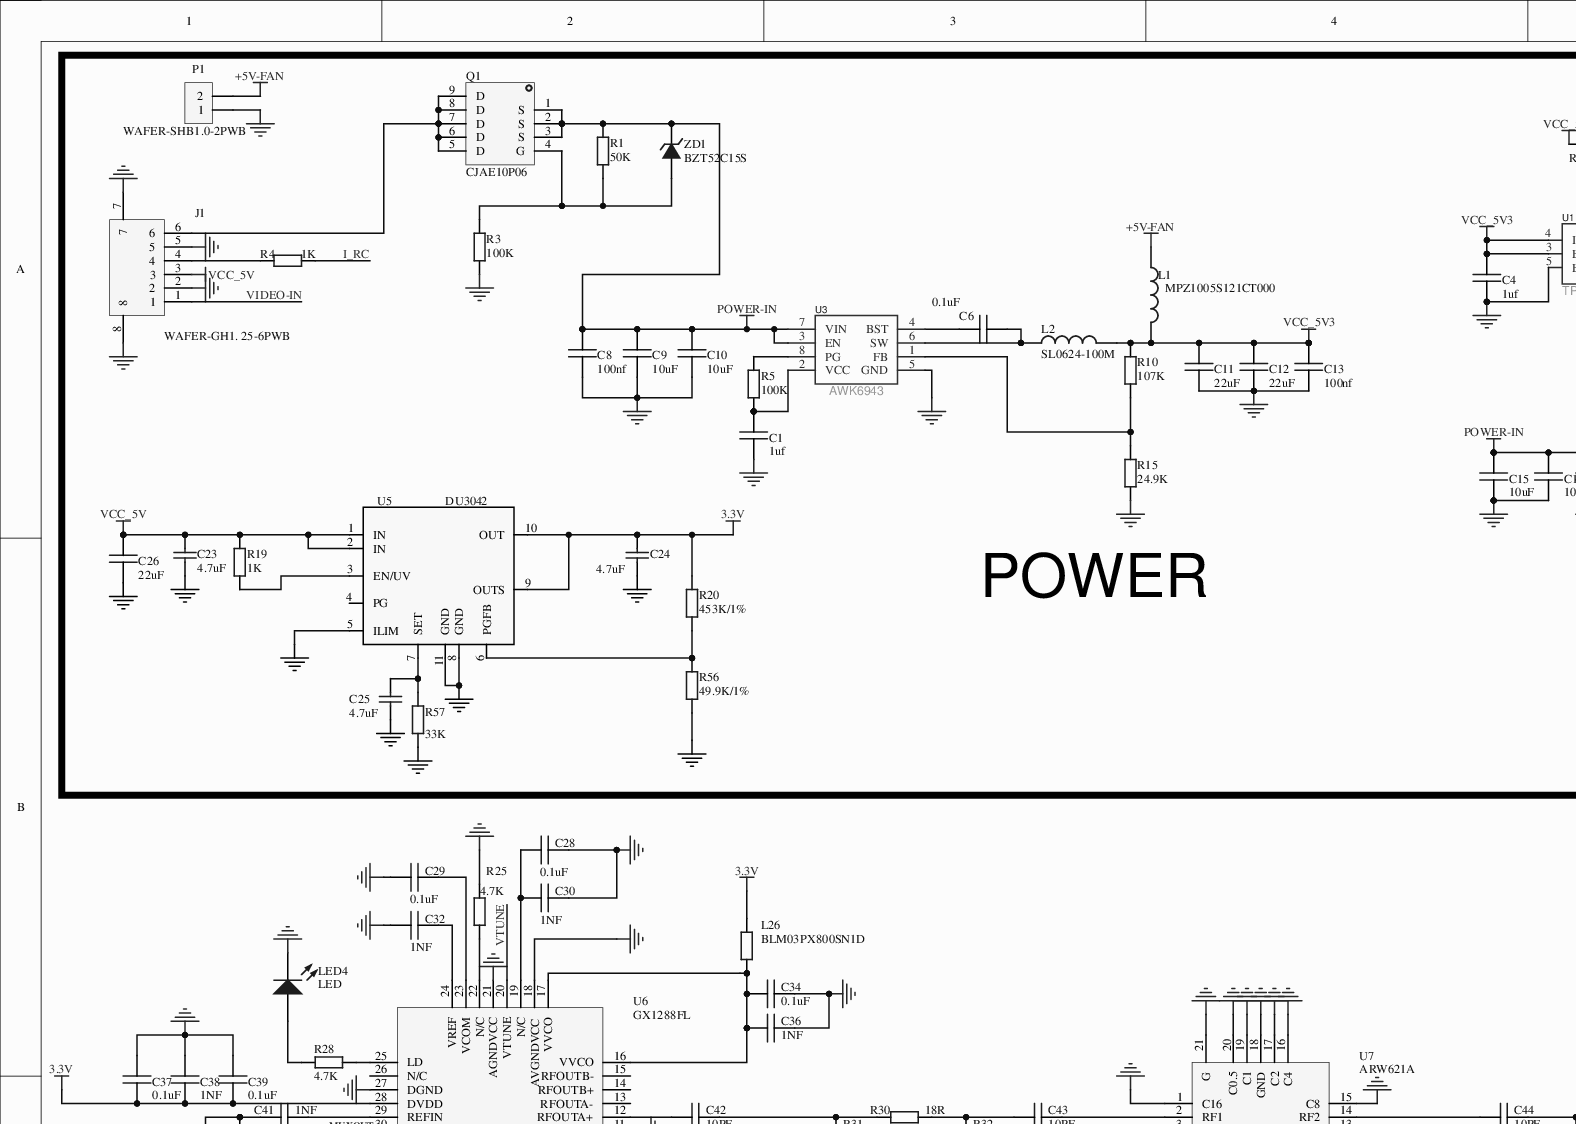
[diagram p0: MISC79034-2.SchDoc, top left]
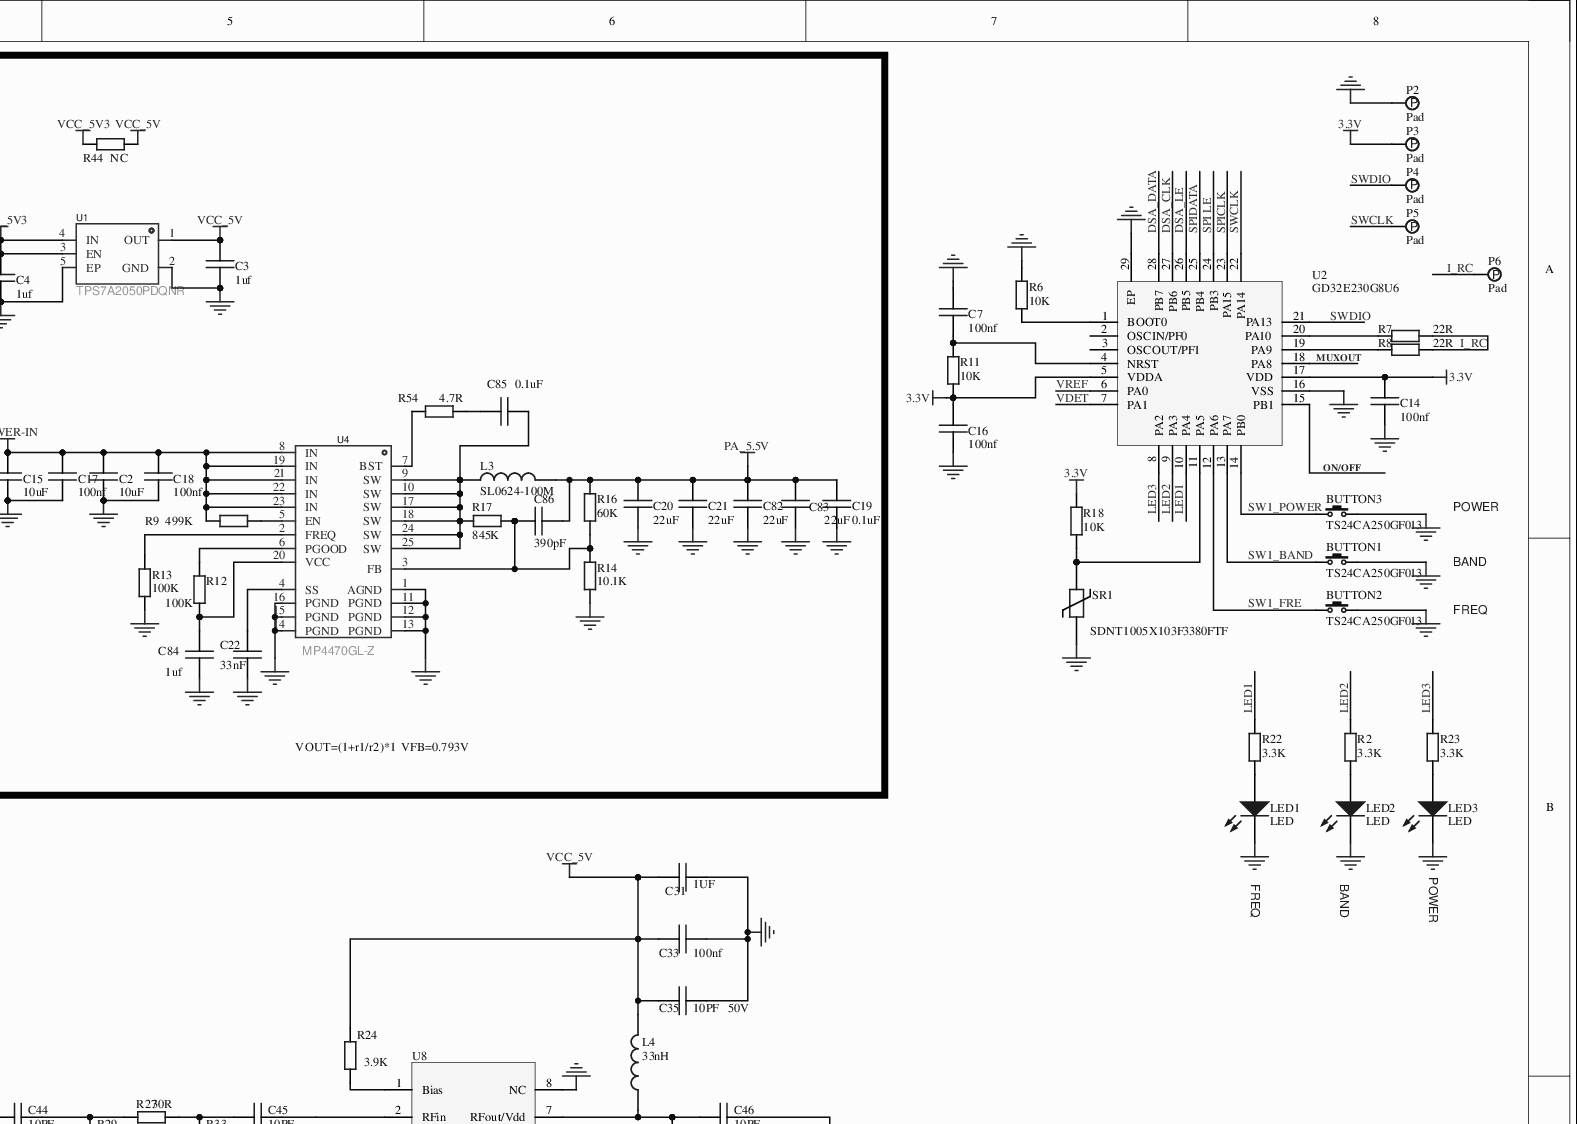
[diagram p1: MISC79034-2.SchDoc, top right]
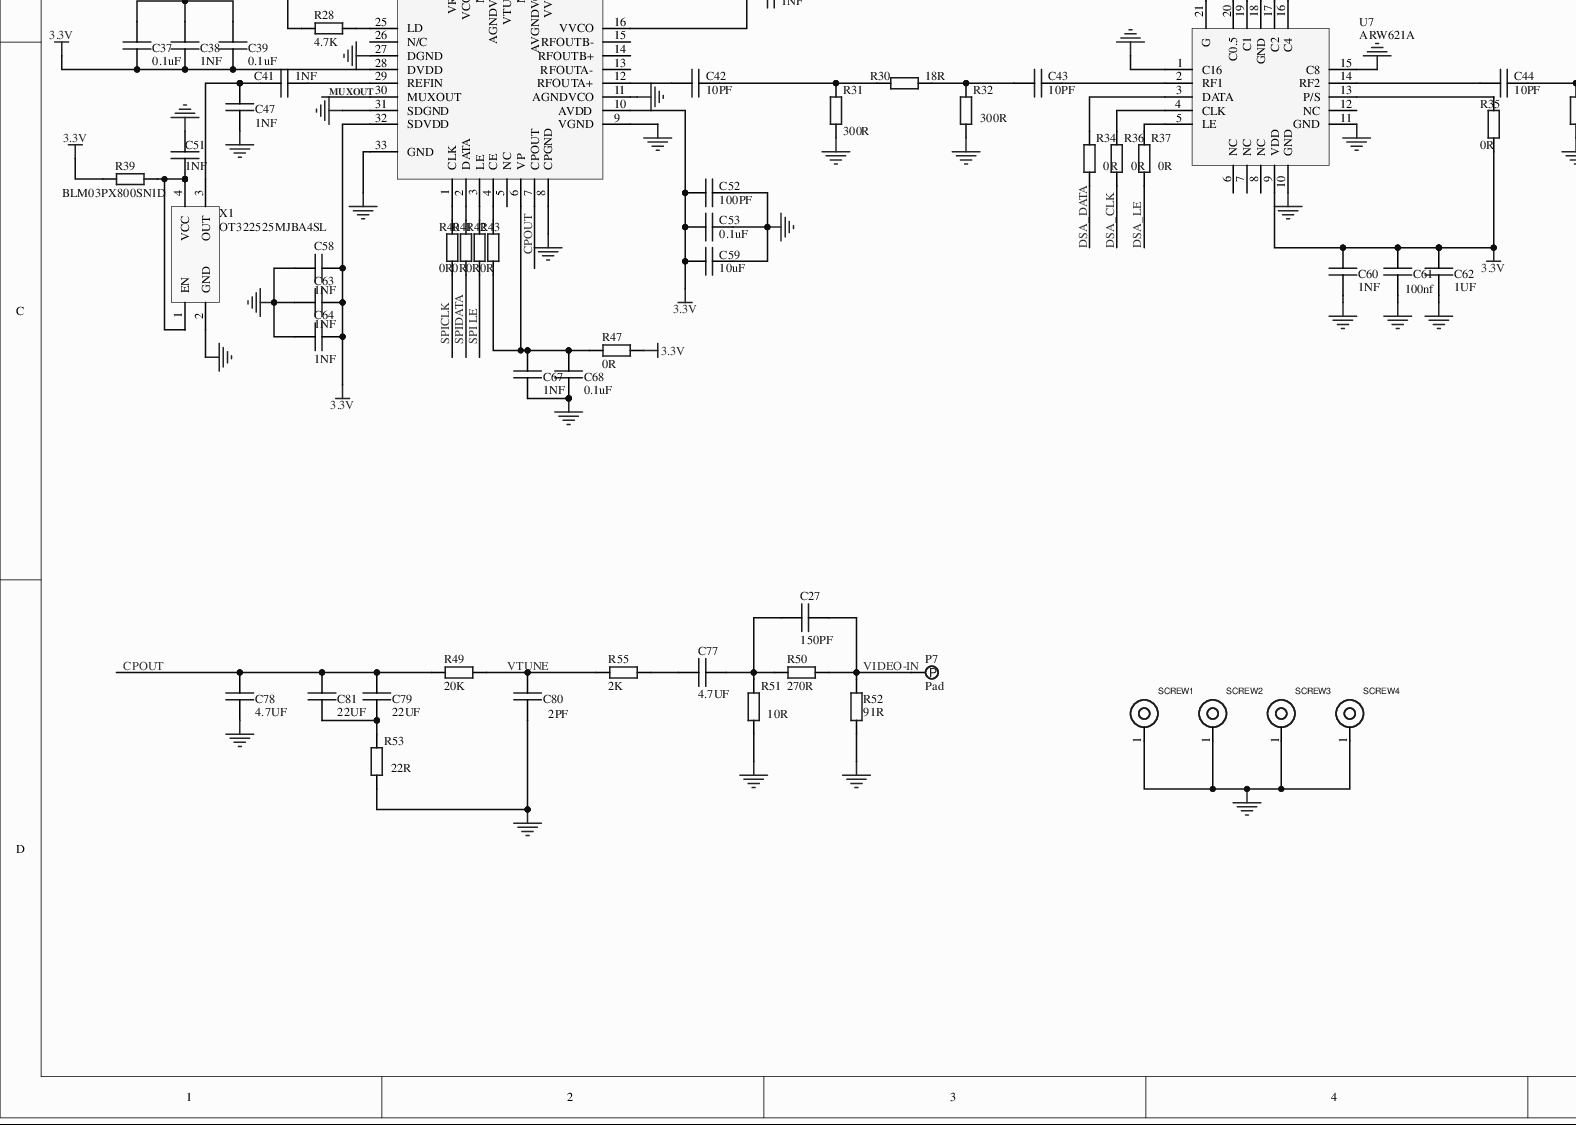
[diagram p2: MISC79034-2.SchDoc, bottom left]
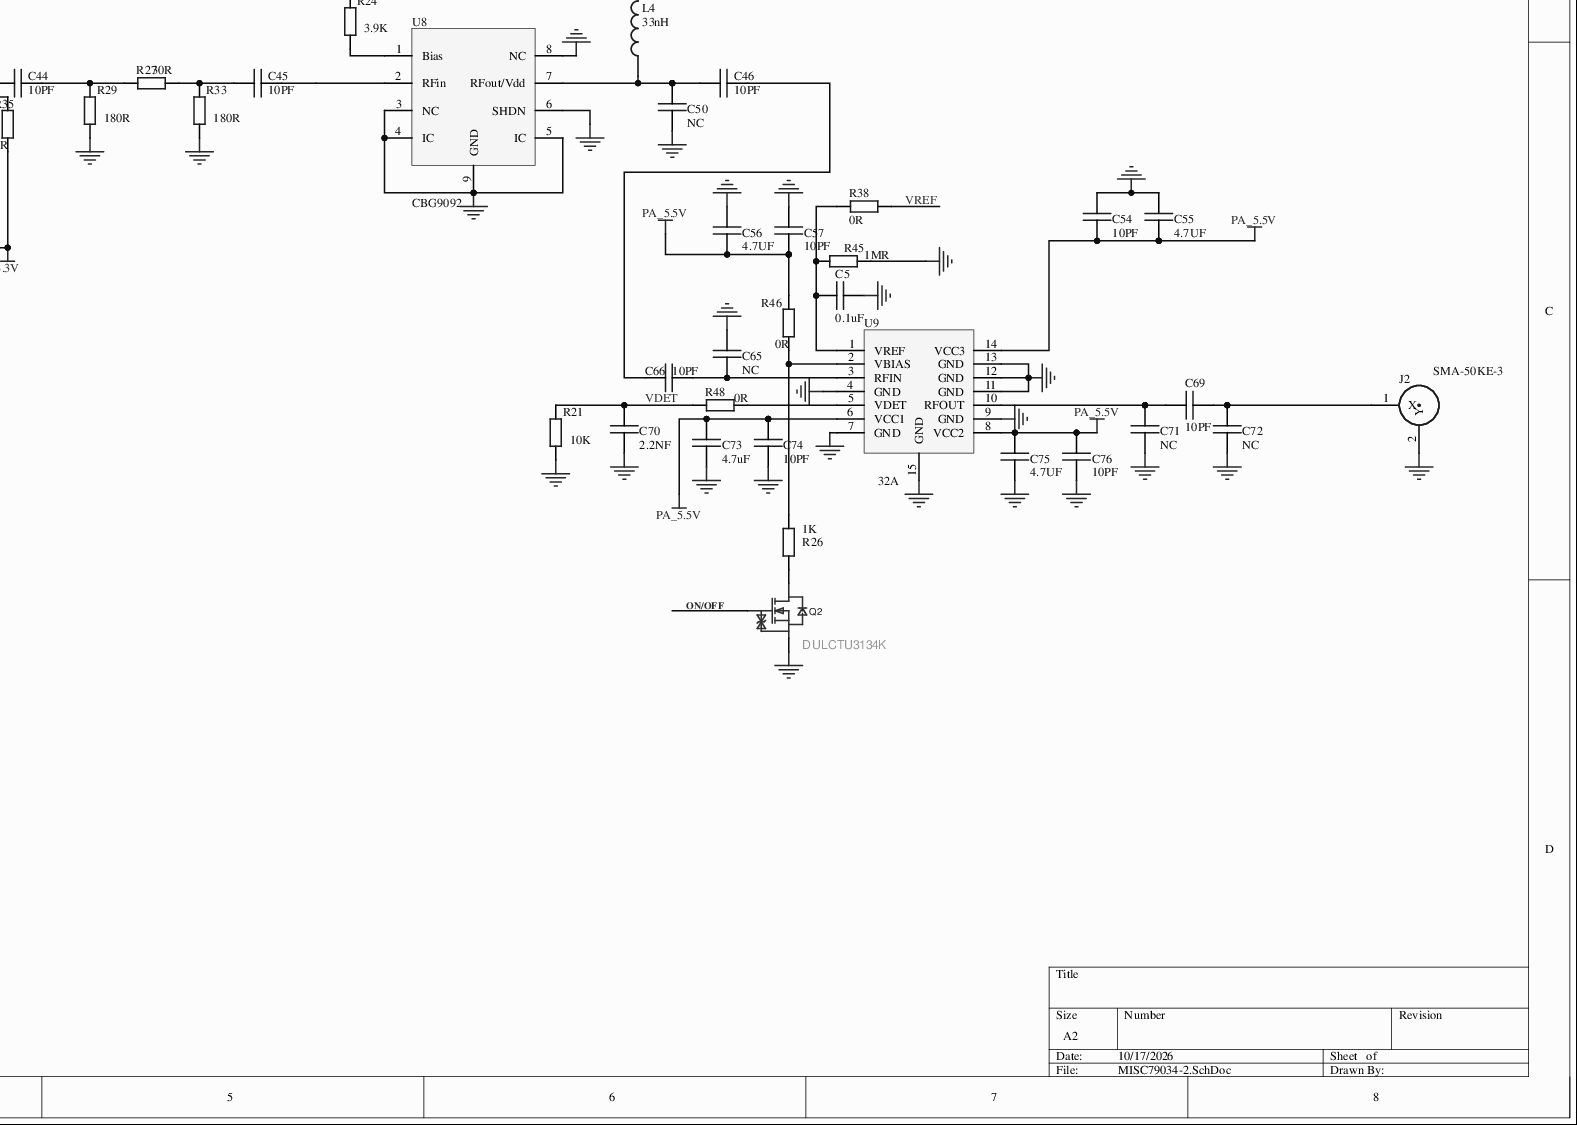
[diagram p3: MISC79034-2.SchDoc, bottom right]
# Altium project MISC79034-33.PrjPCB
1 sheet, 179 parts. Net scope: global (net labels, ports and power ports of the same name join across sheets).
Board file: MISC79034.PcbDoc

## Sheet MISC79034-2.SchDoc
size A2; SheetNumber: 1; SheetTotal: 1

### Parts
BUTTON1  TS24CA250GF013  [SW-SMD_L4.7-W3.5-P3.35-EH]
BUTTON2  TS24CA250GF013  [SW-SMD_L4.7-W3.5-P3.35-EH]
BUTTON3  TS24CA250GF013  [SW-SMD_L4.7-W3.5-P3.35-EH]
C1  1uf  [C0603]
C2  10uF  [C0805]
C3  1uf  [C0603]
C4  1uf  [C0603]
C5  0.1uF  [C0402]
C6  0.1uF  [C0402]
C7  100nf  [C0201]
C8  100nf  [C0402]
C9  10uF  [C0805]
C10  10uF  [C0805]
C11  22uF  [C0603]
C12  22uF  [C0603]
C13  100nf  [C0402]
C14  100nf  [C0201]
C15  10uF  [C0805]
C16  100nf  [C0201]
C17  100nf  [C0402]
C18  100nf  [C0402]
C19  0.1uF  [C0402]
C20  22uF  [C0603]
C21  22uF  [C0603]
C22  33nF  [C0402]
C23  4.7uF  [C0603]
C24  4.7uF  [C0603]
C25  4.7uF  [C0603]
C26  22uF  [C0603]
C27  150PF  [C0402]
C28  0.1uF  [C0201]
C29  0.1uF  [C0201]
C30  1NF  [C0201]
C31  1UF  [C0402]
C32  1NF  [C0201]
C33  100nf  [C0402]
C34  0.1uF  [C0201]
C35  10PF   50V  [C0402]
C36  1NF  [C0201]
C37  0.1uF  [C0201]
C38  1NF  [C0201]
C39  0.1uF  [C0201]
C41  1NF  [C0201]
C42  10PF  [C0402]
C43  10PF  [C0402]
C44  10PF  [C0402]
C45  10PF  [C0402]
C46  10PF  [C0402]
C47  1NF  [C0201]
C50  NC  [C0402]
C51  1NF  [C0201]
C52  100PF  [C0201]
C53  0.1uF  [C0201]
C54  10PF  [C0402]
C55  4.7UF  [C0603]
C56  4.7UF  [C0603]
C57  10PF  [C0402]
C58  1NF  [C0201]
C59  10uF  [C0402]
C60  1NF  [C0402]
C61  100nf  [C0402]
C62  1UF  [C0402]
C63  1NF  [C0201]
C64  1NF  [C0201]
C65  NC  [C0402]
C66  10PF  [C0402]
C67  1NF  [C0201]
C68  0.1uF  [C0201]
C69  10PF  [C0402]
C70  2.2NF  [C0402]
C71  NC  [C0402]
C72  NC  [C0402]
C73  4.7uF  [C0603]
C74  10PF  [C0402]
C75  4.7UF  [C0603]
C76  10PF  [C0402]
C77  4.7UF  [C0402]
C78  4.7UF  [C0402]
C79  22UF  [C0402]
C80  2PF  [C0402]
C81  22UF  [C0402]
C82  22uF  [C0603]
C83  22uF  [C0603]
C84  1uf  [C0603]
C85  0.1uF  [C0402]
C86  390pF  [C0402]
J1  WAFER-GH1. 25-6PWB  [SMD_6P-P1.25_XUNPU_WAFER-GH1.25-6PWB]
J2  SMA-50KE-3  [SMA-FP-945G]
L1  MPZ1005S121CT000  [L0402]
L2  SL0624-100M  [IND-SMD_L7.1-W6.6]
L3  SL0624-100M  [IND-SMD_L7.1-W6.6]
L4  33nH  [L0402]
L26  BLM03PX800SN1D  [L0201]
LED1  LED  [LED0402]
LED2  LED  [LED0402]
LED3  LED  [LED0402]
LED4  LED  [LED0402]
P1  WAFER-SHB1.0-2PWB  [SMD_2P-WAFER-SHB1.0-2PWB]
P2  Pad  [pad]
P3  Pad  [pad]
P4  Pad  [pad]
P5  Pad  [pad]
P6  Pad  [PAD]
P7  Pad  [PAD]
Q1  CJAE10P06  [DFN-8_L3.0-W3.0-P0.65-BL_G48N03D3]
Q2  DULCTU3134K  [SOT-523-3_L1.6-W0.8-P0.50-LS1.6-BR-1]
R1  50K  [R0402]
R2  3.3K  [R0402]
R3  100K  [R0402]
R4  1K  [R0402]
R5  100K  [R0402]
R6  10K  [R0201]
R7  22R  [R0201]
R8  22R  [R0201]
R9  499K  [R0402]
R10  107K  [R0402]
R11  10K  [R0201]
R12  100K  [R0402]
R13  100K  [R0402]
R14  10.1K  [R0402]
R15  24.9K  [R0402]
R16  60K  [R0402]
R17  845K  [R0402]
R18  10K  [R0201]
R19  1K  [R0402]
R20  453K/1%  [R0402]
R21  10K  [R0402]
R22  3.3K  [R0402]
R23  3.3K  [R0402]
R24  3.9K  [R0402]
R25  4.7K  [R0201]
R26  1K  [R0402]
R27  30R  [R0402]
R28  4.7K  [R0201]
R29  180R  [R0402]
R30  18R  [R0402]
R31  300R  [R0402]
R32  300R  [R0402]
R33  180R  [R0402]
R34  0R  [R0402]
R35  0R  [R0402]
R36  0R  [R0402]
R37  0R  [R0402]
R38  0R  [R0402]
R39  BLM03PX800SN1D  [L0201]
R40  0R  [R0201]
R41  0R  [R0201]
R42  0R  [R0201]
R43  0R  [R0201]
R44  NC  [R0402]
R45  1MR  [R0402]
R46  0R  [R0402]
R47  0R  [R0201]
R48  0R  [R0402]
R49  20K  [R0402]
R50  270R  [R0402]
R51  10R  [R0402]
R52  91R  [R0402]
R53  22R  [R0402]
R54  4.7R  [R1206]
R55  2K  [R0402]
R56  49.9K/1%  [R0402]
R57  33K  [R0402]
SCREW1  MARK_4  [M2]  (value not drawn)
SCREW2  MARK_4  [M2]  (value not drawn)
SCREW3  MARK_4  [M2]  (value not drawn)
SCREW4  MARK_4  [M2]  (value not drawn)
SR1  SDNT1005X103F3380FTF  [R0402]
U1  TPS7A2050PDQNR  [X2SON-4_L1.0-W1.0-P0.65-TL-EP]
U2  GD32E230G8U6  [QFN-28_L4.0-W4.0-P0.40-BL-EP2.8]
U3  AWK6943  [QFN-8_L3.0-W3.0-P0.65-BL]
U4  MP4470GL-Z  [QFN-20_L4.0-W3.0_MP9447GL]
U5  DU3042  [WSON-10_L3.0-W3.0-P0.50-BL-EP]
U6  GX1288FL  [QFN-32_L5.0-W5.0-P0.50]
U7  ARW621A  [QFN-20_L4.0-W4.0-P0.50-TL-EP2.2]
U8  CBG9092  [CBG9092]
U9  32A  [AU64XX]
X1  OT322525MJBA4SL  [SMD3225]
ZD1  BZT52C15S  [SOD-323_L1.7-W1.3-LS2.6-RD]

### Blocks framed on the sheet
POWER: C1-C4 C6 C8-C13 C15 C17-C26 C82-C86 J1 L1-L3 P1 Q1 R1 R3-R5 R9 R10 R12-R17 R19 R20 R44 R54 R56 R57 U1 U3-U5 ZD1

### Nets
3.3V: C14.1 C16.1 C24.2 C37.2 C38.1 C39.2 C52.1 C53.2 C58.2 C59.2 C60.2 C61.2 C62.2 C63.2 C64.1 L26.1 P3.1 R11.2 R18.1 R20.1 R35.2 R39.1 R47.2 U2.5(VDDA) U2.17(VDD) U5.9(OUTS) U5.10(OUT) U6.10(AVDD) U6.28(DVDD) U6.32(SDVDD) U7.9(VDD)
+5V-FAN: L1.1 P1.2
GND: BUTTON1.1 BUTTON2.1 BUTTON3.1 C1.2 C2.2 C3.2 C4.2 C5.1 C7.1 C8.2 C9.2 C10.2 C11.2 C12.2 C13.2 C14.2 C15.2 C16.2 C17.2 C18.2 C19.1 C20.2 C21.2 C22.1 C23.1 C24.1 C25.1 C26.2 C28.1 C29.2 C30.2 C31.1 C32.1 C33.1 C34.1 C35.2 C36.2 C37.1 C38.2 C39.1 C47.2 C50.2 C51.1 C52.2 C53.1 C54.2 C55.2 C56.1 C57.1 C58.1 C59.1 C60.1 C61.1 C62.1 C63.1 C64.2 C65.2 C67.2 C68.1 C70.1 C71.1 C72.1 C73.2 C74.2 C75.2 C76.2 C78.2 C80.1 C82.2 C83.2 C84.2 J1.2 J1.5 J1.7 J1.8 J2.2(Y) LED1.2(K) LED2.2(K) LED3.2(K) LED4.2(K) P1.1 P2.1 Q2.2(S) R3.1 R6.1 R13.2 R14.2 R15.2 R21.2 R25.1 R29.2 R31.2 R32.2 R33.2 R45.2 R51.2 R52.2 R53.2 R56.2 R57.1 SCREW1.1 SCREW2.1 SCREW3.1 SCREW4.1 SR1.2 U1.2(GND) U1.5(EP) U2.16(VSS) U2.29(EP) U3.5(GND) U4.1(AGND) U4.11(PGND) U4.12(PGND) U4.13(PGND) U4.14(PGND) U4.15(PGND) U4.16(PGND) U5.5(ILIM) U5.8(GND) U5.11(GND) U6.8(CPGND) U6.9(VGND) U6.11(AGNDVCO) U6.18(AVGNDVCC) U6.21(AGNDVCC) U6.27(DGND) U6.31(SDGND) U6.33(GND) U7.1(C16) U7.10(GND) U7.11(GND) U7.15(C8) U7.16(C4) U7.17(C2) U7.18(GND) U7.19(C1) U7.20(C0.5) U7.21(G) U8.3(NC) U8.4(IC) U8.5(IC) U8.6(SHDN) U8.8(NC) U8.9(GND) U9.4(GND) U9.7(GND) U9.9(GND) U9.11(GND) U9.12(GND) U9.13(GND) U9.15(GND) X1.2(GND)
PA_5.5V: C19.2 C20.1 C21.1 C54.1 C55.1 C56.2 C57.2 C73.1 C74.1 C75.1 C76.1 C82.1 C83.1 C86.1 L3.2 R16.1 R46.1 U9.6(VCC1) U9.8(VCC2) U9.14(VCC3)
POWER-IN: C2.1 C8.1 C9.1 C10.1 C15.1 C17.1 C18.1 Q1.1(S) Q1.2(S) Q1.3(S) R1.2 R9.2 U3.3(EN) U3.7(VIN) U4.8(IN) U4.19(IN) U4.21(IN) U4.22(IN) U4.23(IN) ZD1.2(K)
VCC_5V: C3.1 C23.2 C26.1 C31.2 C33.2 C35.1 J1.3 L4.2 R19.2 R24.1 R44.2 U1.1(OUT) U5.1(IN) U5.2(IN)
VCC_5V3: C4.1 C11.1 C12.1 C13.1 L1.2 L2.2 R10.1 R44.1 U1.3(EN) U1.4(IN)
CPOUT: C78.1 C79.2 C81.2 R49.1 U6.7(CPOUT)
DSA_CLK: R36.2 U2.27(PB6)
DSA_DATA: R34.2 U2.28(PB7)
DSA_LE: R37.2 U2.26(PB5)
I_RC: P6.1 R4.2 R7.2 R8.2
LED1: R22.1 U2.10(PA4)
LED2: R2.1 U2.9(PA3)
LED3: R23.1 U2.8(PA2)
MUXOUT: U2.18(PA8) U6.30(MUXOUT)
ON/OFF: Q2.1(G) U2.15(PB1)
SPI LE: R42.2 U2.24(PB3)
SPICLK: R40.2 U2.23(PA15)
SPIDATA: R41.2 U2.25(PB4)
SW1_BAND: BUTTON1.2 U2.13(PA7)
SW1_FRE: BUTTON2.2 U2.12(PA6)
SW1_POWER: BUTTON3.2 U2.14(PB0)
SWCLK: P5.1 U2.22(PA14)
SWDIO: P4.1 U2.21(PA13)
VDET: C70.2 R21.1 R48.1 U2.7(PA1)
VIDEO-IN: C27.1 J1.1 P7.1 R50.2 R52.1
VREF: R38.1 U2.6(PA0)
VTUNE: C80.2 R49.2 R55.1 U6.20(VTUNE)
NetC1_1: C1.1 R5.1 U3.2(VCC)
NetC5_2: C5.2 R38.2 R45.1 U9.1(VREF)
NetC6_1: C6.1 U3.4(BST)
NetC6_2: C6.2 L2.1 U3.6(SW)
NetC7_2: C7.2 R11.1 U2.4(NRST)
NetC22_2: C22.2 U4.4(SS)
NetC25_2: C25.2 R57.2 U5.7(SET)
NetC27_2: C27.2 C77.1 R50.1 R51.1
NetC28_2: C28.2 C30.1 U6.19(N/C)
NetC29_1: C29.1 U6.23(VCOM)
NetC32_2: C32.2 U6.24(VREF)
NetC34_2: C34.2 C36.1 L26.2 U6.16(VVCO) U6.17(VVCO)
NetC41_1: C41.1 U6.29(REFIN)
NetC41_2: C41.2 C47.1 X1.3(OUT)
NetC42_1: C42.1 U6.12(RFOUTA+)
NetC42_2: C42.2 R30.1 R31.1
NetC43_1: C43.1 R30.2 R32.1
NetC43_2: C43.2 U7.2(RF1)
NetC44_1: C44.1 U7.14(RF2)
NetC44_2: C44.2 R27.1 R29.1
NetC45_1: C45.1 R27.2 R33.1
NetC45_2: C45.2 U8.2(RFin)
NetC46_1: C46.1 C50.1 L4.1 U8.7(RFout/Vdd)
NetC46_2: C46.2 C66.2
NetC51_2: C51.2 R39.2 X1.1(EN) X1.4(VCC)
NetC65_1: C65.1 C66.1 U9.3(RFIN)
NetC67_1: C67.1 C68.2 R43.2 R47.1 U6.6(VP)
NetC69_1: C69.1 C71.2 U9.10(RFOUT)
NetC69_2: C69.2 C72.2 J2.1(X)
NetC77_2: C77.2 R55.2
NetC79_1: C79.1 C81.1 R53.1
NetC84_1: C84.1 R12.2 U4.20(VCC)
NetC85_1: C85.1 R54.1
NetC85_2: C85.2 L3.1 R17.1 U4.9(SW) U4.10(SW) U4.17(SW) U4.18(SW) U4.24(SW) U4.25(SW)
NetC86_2: C86.2 R14.1 R16.2 R17.2 U4.3(FB)
NetJ1_4: J1.4 R4.1
NetJ1_6: J1.6 Q1.5(D) Q1.6(D) Q1.7(D) Q1.8(D) Q1.9(D)
NetLED1_1: LED1.1(A) R22.2
NetLED2_1: LED2.1(A) R2.2
NetLED3_1: LED3.1(A) R23.2
NetLED4_1: LED4.1(A) R28.1
NetQ1_4: Q1.4(G) R1.1 R3.2 ZD1.1(A)
NetQ2_3: Q2.3(D) R26.2
NetR5_2: R5.2 U3.8(PG)
NetR6_2: R6.2 U2.1(BOOT0)
NetR7_1: R7.1 U2.20(PA10)
NetR8_1: R8.1 U2.19(PA9)
NetR9_1: R9.1 U4.5(EN)
NetR10_2: R10.2 R15.1 U3.1(FB)
NetR12_1: R12.1 U4.6(PGOOD)
NetR13_1: R13.1 U4.2(FREQ)
NetR18_2: R18.2 SR1.1 U2.11(PA5)
NetR19_1: R19.1 U5.3(EN/UV)
NetR20_2: R20.2 R56.1 U5.6(PGFB)
NetR24_2: R24.2 U8.1(Bias)
NetR25_2: R25.2 U6.22(N/C)
NetR26_1: R26.1 R46.2 U9.2(VBIAS)
NetR28_2: R28.2 U6.25(LD)
NetR34_1: R34.1 U7.3(DATA)
NetR35_1: R35.1 U7.13(P/S)
NetR36_1: R36.1 U7.4(CLK)
NetR37_1: R37.1 U7.5(LE)
NetR40_1: R40.1 U6.1(CLK)
NetR41_1: R41.1 U6.2(DATA)
NetR42_1: R42.1 U6.3(LE)
NetR43_1: R43.1 U6.4(CE)
NetR48_2: R48.2 U9.5(VDET)
NetR54_2: R54.2 U4.7(BST)

Not connected (* = marked no-connect by the designer): U2 2(OSCIN/PF0) 3(OSCOUT/PF1); U5 4(PG); U6 5(NC) 13(RFOUTA-) 14(RFOUTB+) 15(RFOUTB-) 26(N/C); U7 6(NC) 7(NC) 8(NC) 12(NC)

### Notes on the sheet
- POWER
- BAND
- FREQ
- VOUT=(1+r1/r2)*1  VFB=0.793V

### Library data of the parts
BUTTON1-BUTTON3 = TSW 3x6: 3x6 tact switch; BOM名称: 3x6 tact switch
C1-C6 C9-C12 C15 C19-C22 C26-C32 C34-C39 C41-C47 C50-C60 C62-C86 = 100nf
C23-C25 = C: Chip capacitor; BOM名称: Non-polarized chip capacitor
L1-L4 = L-AL: Color-ring inductor; BOM名称: Color-ring inductor
L26 R1-R57 = R: Chip resistor; BOM名称: Chip resistor
LED1-LED4 = LED0: Light-emitting diode; Published: 8-Jun-2000; LatestRevisionDate: 08-Jul-2005; LatestRevisionNote: Mech Layer 1 removed.; PackageReference: LED-0; Publisher: Altium Limited
P1 = Header 2: 2P connector; BOM名称: 2P connector
Q2 = 2N7002T_C5224243: Symbol: 2N7002T_C5224243
SCREW1-SCREW4 = MARK_4: MARK Symble; RK_PN: MARK01; Priority: A; Created_by: CZD; Source_Path: RK3399_BOX_SCH_V1.0_20180521.DSN; Value: SCREEW; Part_Type: MARK; PCB DECAL: MARK
U3 = TPS54327DDAR: Symbol: TPS54327DDAR
U5 = DAC53202RTER: No Description Available; Mfr_Name: Texas Instruments; Type: Data Acquisition; RefDes: RefDes
U9 = GCM3527(3.3G-3.8G)
X1 = XTAL-ACT-4P: 4-pin active crystal oscillator; 版权归属: Copyright: COMPANY_B; BOM名称: 4-pin active crystal oscillator
ZD1 = 1N4733: 5.1V/1W Zener diode; BOM名称: 5.1V/1W Zener diode
U1 = TPS7A2050PDQNR: Symbol: TPS7A2050PDQNR
U4 = MP4470GL-Z: Symbol: MP4470GL-Z